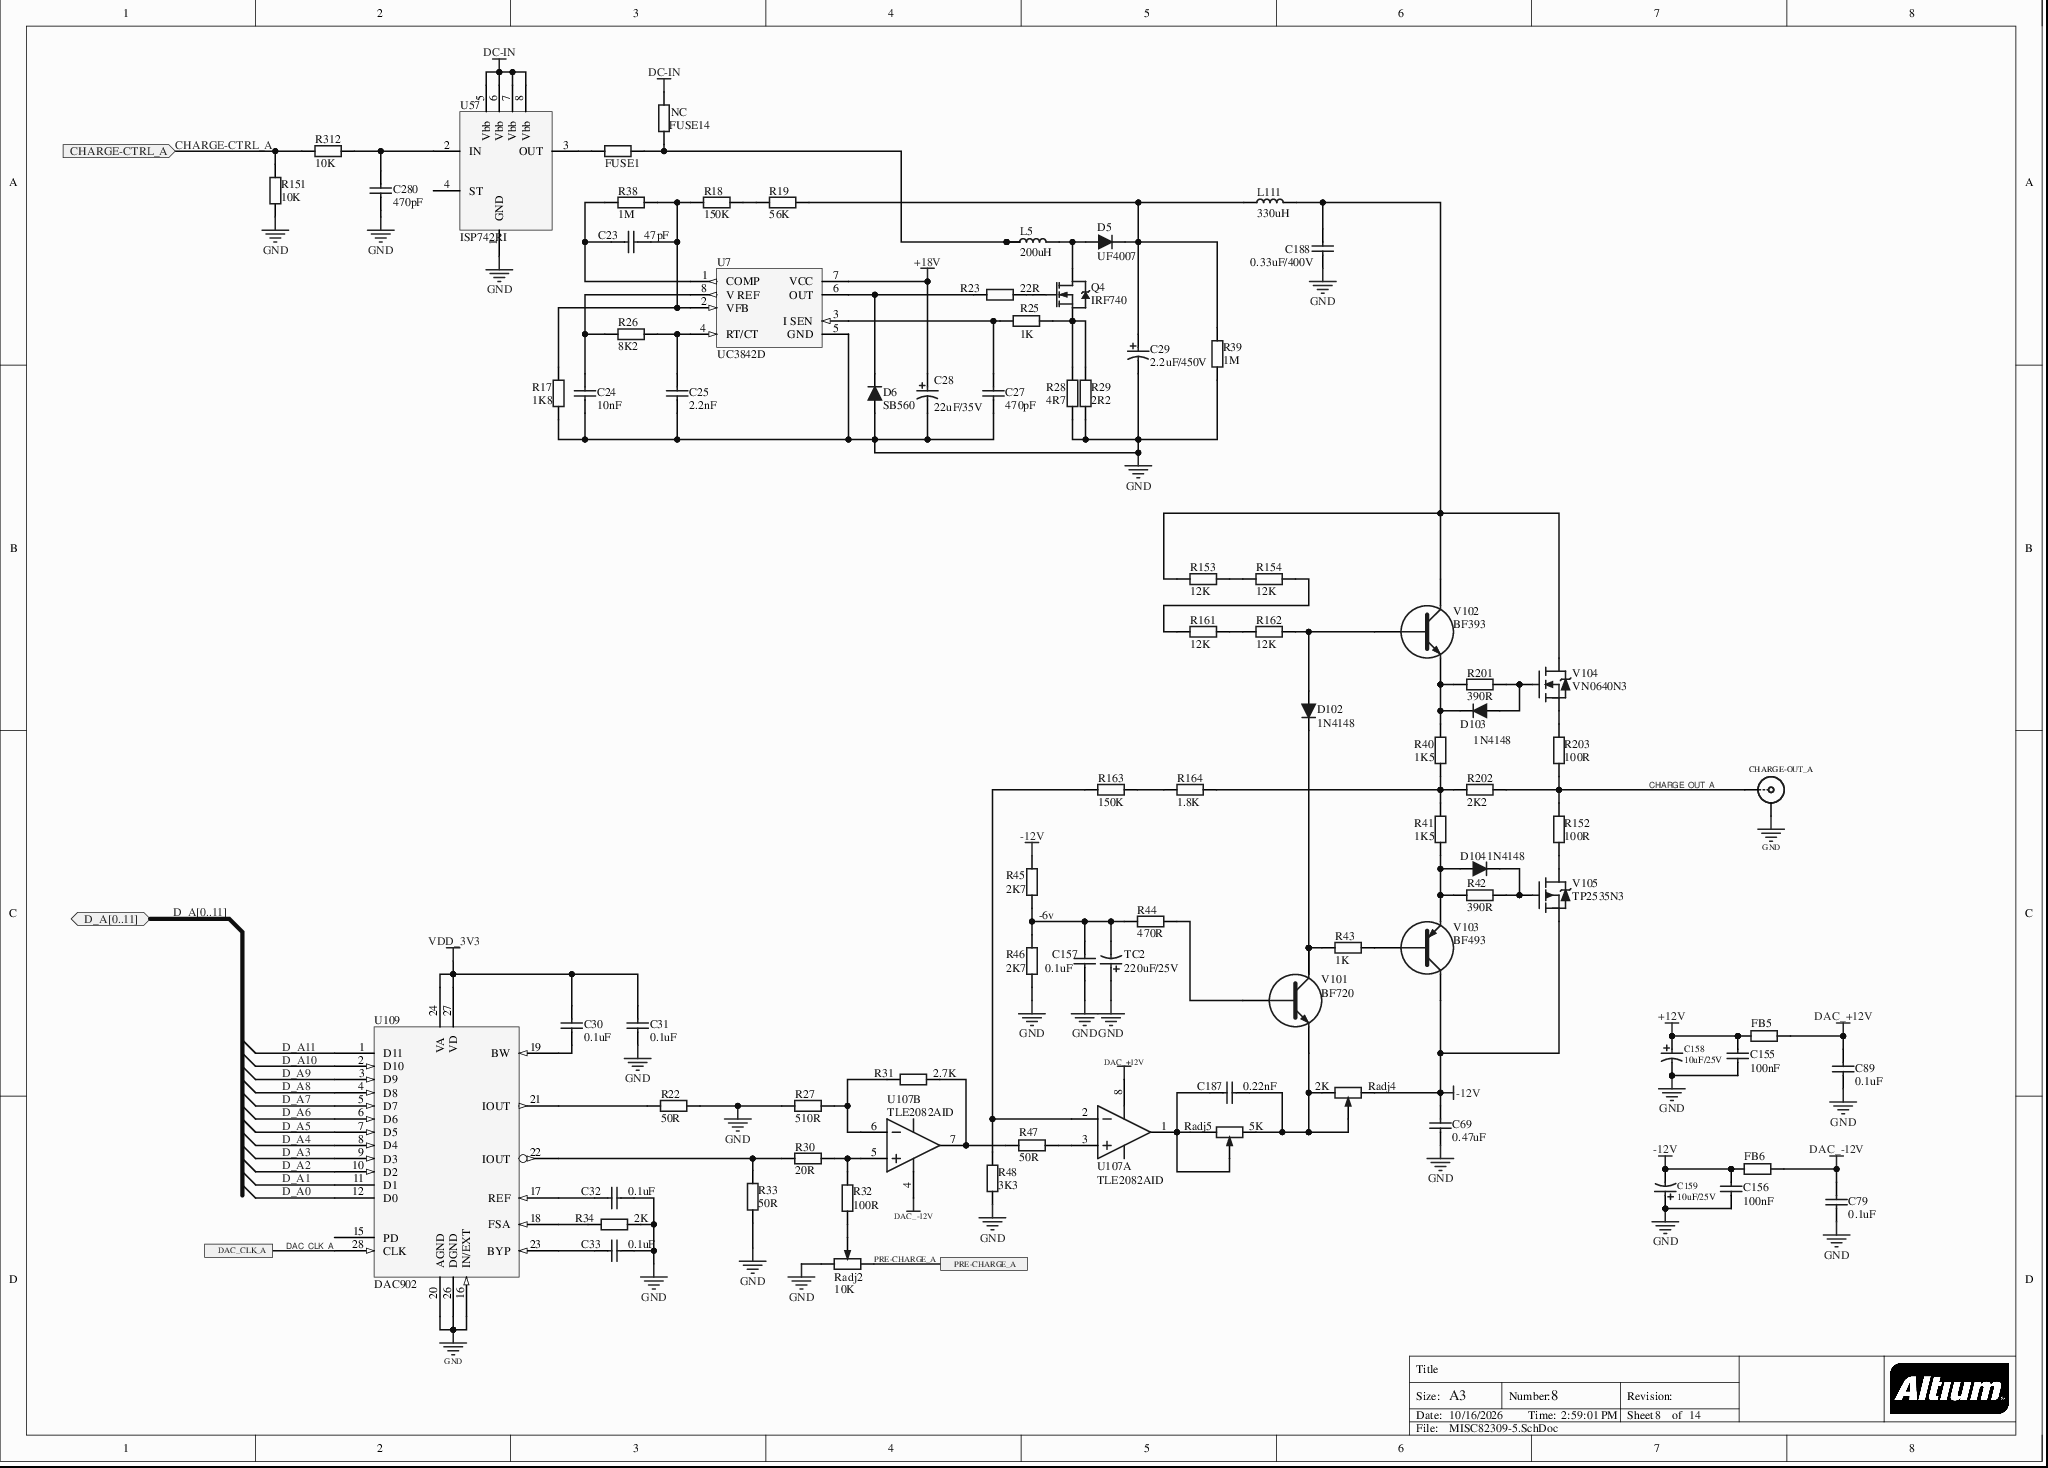
[diagram p0: MISC82309-5.SchDoc]
# Altium project MISC82309-16.PrjPcb (part 4 of 6)

## Sheet MISC82309-5.SchDoc
size A3; DocumentNumber: 8; SheetNumber: 8; SheetTotal: 14

### Parts
C23  47pF  [C1206]
C24  10nF  [C1206]
C25  2.2nF  [C1206]
C27  470pF  [C1206]
C28  22uF/35V  [E6.3X5.4]
C29  2.2uF/450V  [CAP-EL-10X13_5-5]
C30  0.1uF  [CAP_0805]
C31  0.1uF  [CAP_0805]
C32  0.1uF  [CAP_0805]
C33  0.1uF  [CAP_0805]
C69  0.47uF  [C1206]
C79  0.1uF  [C0805]
C89  0.1uF  [C0805]
C155  100nF  [C0805]
C156  100nF  [C0805]
C157  0.1uF  [CAP_0805]
C158  10uF/25V  [E5X5.4]
C159  10uF/25V  [E5X5.4]
C187  0.22nF  [CAP_0805]
C188  0.33uF/400V  [CBB-400V-10mm]
C280  470pF  [C0603]
CHARGE-OUT_A  SMB  [SMB_V-RJ45]  (value not drawn)
D5  UF4007  [DO-41 - 10.46mm]
D6  SB560  [SB560]
D102  1N4148  [DO-213AA]
D103  1N4148  [DO-213AA]
D104  1N4148  [DO-213AA]
FB5  60  [SMD0805-L]  (value not drawn)
FB6  60  [SMD0805-L]  (value not drawn)
FUSE1  ASMD050-1812(30V,0.5A)  [SMD1812-Fuse]  (value not drawn)
FUSE14  value NC  [SMD1812-Fuse]  (hidden comment: ASMD050-1812(30V,0.5A))
L5  200uH  [L200/1.4A]
L111  330uH  [L-9x12]
Q4  IRF740  [TO220V1]
R17  1K8  [R1206]
R18  150K  [R1206]
R19  56K  [R1206]
R22  50R  [RES_0805]
R23  22R  [R1206]
R25  1K  [R1206]
R26  8K2  [R1206]
R27  510R  [RES_0805]
R28  4R7  [R1206]
R29  2R2  [R1206]
R30  20R  [RES_0805]
R31  2.7K  [RES_0805]
R32  100R  [RES_0805]
R33  50R  [RES_0805]
R34  2K  [RES_0805]
R38  1M  [R1206]
R39  1M  [R1206]
R40  1K5  [R1206]
R41  1K5  [R1206]
R42  390R  [R1206]
R43  1K  [R1206]
R44  470R  [RES_0805]
R45  2K7  [RES_0805]
R46  2K7  [RES_0805]
R47  50R  [RES_0805]
R48  3K3  [RES_0805]
R151  10K  [R0603]
R152  100R  [R1206]
R153  12K  [R1206]
R154  12K  [R1206]
R161  12K  [R1206]
R162  12K  [R1206]
R163  150K  [R1206]
R164  1.8K  [R1206]
R201  390R  [R1206]
R202  2K2  [R1206]
R203  100R  [R1206]
R312  10K  [R0603]
Radj2  10K  [Radj]
Radj4  2K  [Radj]
Radj5  5K  [Radj]
TC2  220uF/25V  [E8X10,2]
U7  UC3842D  [SOIC-8]
U57  ISP742RI  [P-DSO-8]
U107  TLE2082AID  [SOIC-8]  (parts A,B of 2)
U109  DAC902  [SOP127P1020X265-28N]
V101  BF720  [SOT223]
V102  BF393  [TO-92]
V103  BF493  [TO-92]
V104  VN0640N3  [TO-92]
V105  TP2535N3  [TO-92]

### Ports
CHARGE-CTRL_A (in), D_A[0..11] (bidir), DAC_CLK_A, PRE-CHARGE_A

### Nets
+12V: C155.1 C158.1 FB5.1
+18V: C28.1 U7.7(VCC)
-12V: C69.1 C156.1 C159.2 FB6.1 R45.1 Radj4.3 V103.3(C) V105.3(D)
DAC_+12V: C89.2 FB5.2 U107.8
DAC_-12V: C79.2 FB6.2 U107.4
DC-IN: FUSE14.1 U57.5(Vbb) U57.6(Vbb) U57.7(Vbb) U57.8(Vbb)
GND: C24.2 C25.2 C27.2 C28.2 C29.2 C31.2 C32.2 C33.1 C69.2 C79.1 C89.1 C155.2 C156.2 C157.2 C158.2 C159.1 C188.1 C280.1 CHARGE-OUT_A.2(Y) D6.1 R17.1 R22.2 R27.1 R28.1 R29.1 R33.1 R34.2 R39.1 R46.2 R48.1 R151.1 Radj2.3 TC2.1 U7.5(GND) U57.1(GND) U109.16(IN/EXT) U109.20(AGND) U109.26(DGND)
VDD_3V3: C30.1 C31.1 U109.24(VA) U109.27(VD)
CHARGE-CTRL_A: R151.2 R312.2 ; port CHARGE-CTRL_A
CHARGE_OUT_A: CHARGE-OUT_A.1(X) R152.1 R202.2 R203.2
D_A0: U109.12(D0)
D_A1: U109.11(D1)
D_A2: U109.10(D2)
D_A3: U109.9(D3)
D_A4: U109.8(D4)
D_A5: U109.7(D5)
D_A6: U109.6(D6)
D_A7: U109.5(D7)
D_A8: U109.4(D8)
D_A9: U109.3(D9)
D_A10: U109.2(D10)
D_A11: U109.1(D11)
DAC_CLK_A: U109.28(CLK) ; port DAC_CLK_A
PRE-CHARGE_A: Radj2.1 ; port PRE-CHARGE_A
NetC23_1: C23.1 R17.2 R18.1 R38.2 U7.2(VFB)
NetC23_2: C23.2 R38.1 U7.1(COMP)
NetC24_1: C24.1 R26.1 U7.8(V_REF)
NetC25_1: C25.1 R26.2 U7.4(RT/CT)
NetC27_1: C27.1 R25.1 U7.3(I_SEN)
NetC29_1: C29.1 D5.2 L111.1 R19.2 R39.2
NetC30_2: C30.2 U109.19(BW)
NetC32_1: C32.1 U109.17(REF)
NetC33_2: C33.2 U109.23(BYP)
NetC157_1: C157.1 R44.2 R45.2 R46.1 TC2.2
NetC187_1: C187.1 Radj4.1 Radj4.2 Radj5.3 V101.3(E)
NetC187_2: C187.2 Radj5.1 Radj5.2 U107.1
NetC188_2: C188.2 L111.2 R153.2 V102.3(C) V104.3(D)
NetC280_2: C280.2 R312.1 U57.2(IN)
NetD5_1: D5.1 L5.2 Q4.2(D)
NetD6_2: D6.2 R23.1 U7.6(OUT)
NetD102_1: D102.1 R162.1 V102.2(B)
NetD102_2: D102.2 R43.2 V101.2(C) V101.4(C)
NetD103_1: D103.1 R201.2 V104.2(G)
NetD103_2: D103.2 R40.1 R201.1 V102.1(E)
NetD104_1: D104.1 R41.2 R42.1 V103.1(E)
NetD104_2: D104.2 R42.2 V105.2(G)
NetFUSE1_1: FUSE1.1 U57.3(OUT)
NetFUSE1_2: FUSE1.2 FUSE14.2 L5.1 L5.3
NetQ4_1: Q4.1(G) R23.2
NetQ4_3: Q4.3(S) R25.2 R28.2 R29.2
NetR18_2: R18.2 R19.1
NetR22_1: R22.1 U109.21(IOUT)
NetR27_2: R27.2 R31.1 U107.6
NetR30_1: R30.1 R33.2 U109.22(IOUT)
NetR30_2: R30.2 R32.2 U107.5
NetR31_2: R31.2 R47.1 U107.7
NetR32_1: R32.1 Radj2.2
NetR34_1: R34.1 U109.18(FSA)
NetR40_2: R40.2 R41.1 R164.1 R202.1
NetR43_1: R43.1 V103.2(B)
NetR44_1: R44.1 V101.1(B)
NetR47_2: R47.2 U107.3
NetR48_2: R48.2 R163.2 U107.2
NetR152_2: R152.2 V105.1(S)
NetR153_1: R153.1 R154.2
NetR154_1: R154.1 R161.2
NetR161_1: R161.1 R162.2
NetR163_1: R163.1 R164.2
NetR203_1: R203.1 V104.1(S)

Not connected (* = marked no-connect by the designer): U57 4(ST); U109 15(PD)

### Buses and harness runs
bus D_A[0..11] = port D_A[0..11]

### Notes on the sheet
- (near R45) -6v
- Title
- Size:
- Date:
- A3
- Number:
- Time:
- Revision:
- Sheet
- of
- File:

### Library data of the parts
C23 = CAP_47pF: Capacitor 47pF; Value: 47pF
C24 = CAP_10nF: Capacitor 10nF; Value: 10nF
C25 = CAP_2.2nF: Capacitor 2.2nF; Value: 2.2nF
C27 = CAP_470pF: Capacitor 470pF; Value: 470pF
C28 = CAP_POLAR_22uF_35V: Polar Capacitor 22uF 35V; Value: 22uF/35V
C29 = CAP_POLAR_2.2uF_450V: Polar Capacitor 222uF 450V; Value: 2.2uF/450V
C30-C33 C157 = CAP_0.1uF: Capacitor 0.1uF; Value: 0.1uF
C69 = CAP_0.47uF: Capacitor 0.47uF; Value: 0.47uF
C79 C89 = CAP_1206: Capacitor; value: 0.1uF
C155 = CAP_0.1uF: value: 470pF
C156 C280 = CAP_0.1uF
  C156: value: 100nF
  C280: value: 470pF
C158 C159 = CAP_POLAR_1: Polar Capacitor
C187 = CAP_0.22nF: Capacitor 0.22nF; Value: 0.22nF
C188 = CAP_CBB_0.33uF_400V: CBB Capacitor 0.33uF 400V; Value: 0.33uF/400V
CHARGE-OUT_A = SMB: SMB Straight Connector; LatestRevisionDate: 17-Jul-2002; LatestRevisionNote: Re-released for DXP Platform.; PCB DECAL: SMB_V-RJ45; Comment_1: SMB; Publisher: Altium Limited
FB5 FB6 = FB: Res; value: 10K
FUSE1 = FUSE: Res; Value: 30V/500mA
FUSE14 = FUSE: Res
L5 = Toroidal Inductor
L111 = Power Inductance: Value: 330uH
Q4 = IRF740: HEXFET N-Channel Power MOSFET; Note: Pin 2 is electrically connected to pin 4.; Published: 8-Jun-2000; LatestRevisionDate: 17-Jul-2002; LatestRevisionNote: Re-released for DXP Platform.; DatasheetVersion: PD-9.375H; PackageVersion: Feb-1997; PackageReference: TO-220AB; PackageDescription: TO, Thru-Hole, Vertical, Heatsink Mounted; 3 In-Line Leads; Pitch 2.54 mm; ComponentLink1Description: Manufacturer Link; ComponentLink1URL: http://www.irf.com/; ComponentLink2Description: Datasheet; ComponentLink2URL: http://www.irf.com/product-info/datasheets/data/irf740.pdf; Publisher: Altium Limited
R17 = Res_1K8: Resistance 1.8K; value: 1K8
R18 R163 = Res_150K: Resistance 150K; value: 150K
R19 = Res_68K: Resistance 68K; value: 56K
R22 R33 R47 = Res_50R: Resistance 50R; value: 50R
R23 = Res_22R: Resistance 22R; value: 22R
R25 R43 = Res_1K: Resistance 1K; value: 1K
R26 = Res_8K2: Resistance 8.2K; value: 8K2
R27 R44 = Res_470R: Resistance 470R
  R27: value: 510R
  R44: value: 470R
R28 = Res_4R7: Resistance 4.7R; value: 4R7
R29 = Res_2R2: Resistance 2R2; value: 2R2
R30 R34 = Res_20R: Resistance 20R
  R30: value: 20R
  R34: value: 2K
R31 R164 = Res_2K: Resistance 2K
  R31: value: 2.7K
  R164: value: 1.8K
R32 R152 R203 = Res_100R: Resistance 100R; value: 100R
R38 R39 = Res_1M: Resistance 1M; value: 1M
R40 R41 = Res_1K5: Resistance 1.5K; value: 1K5
R42 R201 = Res_390R: Resistance 390R; value: 390R
R45 R46 = Res_2K7: Resistance 2.7K; value: 2K7
R48 = Res_3K3: Resistance 3.3K; value: 3K3
R151 R312 = Res2: Resistor; Published: 8-Jun-2000; LatestRevisionDate: 17-Jul-2002; LatestRevisionNote: Re-released for DXP Platform.; PackageReference: AXIAL-0.4; Value: 10K; Publisher: Altium Limited
R153 R154 R161 R162 = Res_12K: Resistance 12K; value: 12K
R202 = Res_2K2: Resistance 2.2K; value: 2K2
Radj2 = Res_Adj_10K: Value: 10K
Radj4 = Res_Adj_2K: Value: 2K
Radj5 = Res_Adj_5K: Value: 5K
TC2 = CAP_POLAR_220uF_25V: Polar Capacitor 220uF 25V; Value: 220uF/25V
U7 = UC3842N: Current Mode PWM Controller; PackageReference: SOIC-8
U57 = I742RI
U107 = TLE2082AID: EXCALIBUR HIGH-SPEED JFET-INPUT  OPERATIONAL AMPLIFIERS
V101 = BF720: NPN high-voltage transistors
V102 = BF393: NPN High Voltage Transistor
V103 = BF493: PNP High Voltage Transistor
D6 = SB560: Supplier 1: Newark; Supplier Part Number 1: 05R5713
U109 = DAC902: Supplier 1: Digi-Key; Supplier Part Number 1: DAC902UG4-ND

## Sheet MISC82309-6.SchDoc
size A3; DocumentNumber: 9; Revision: 1.0; SheetNumber: 9; SheetTotal: 14
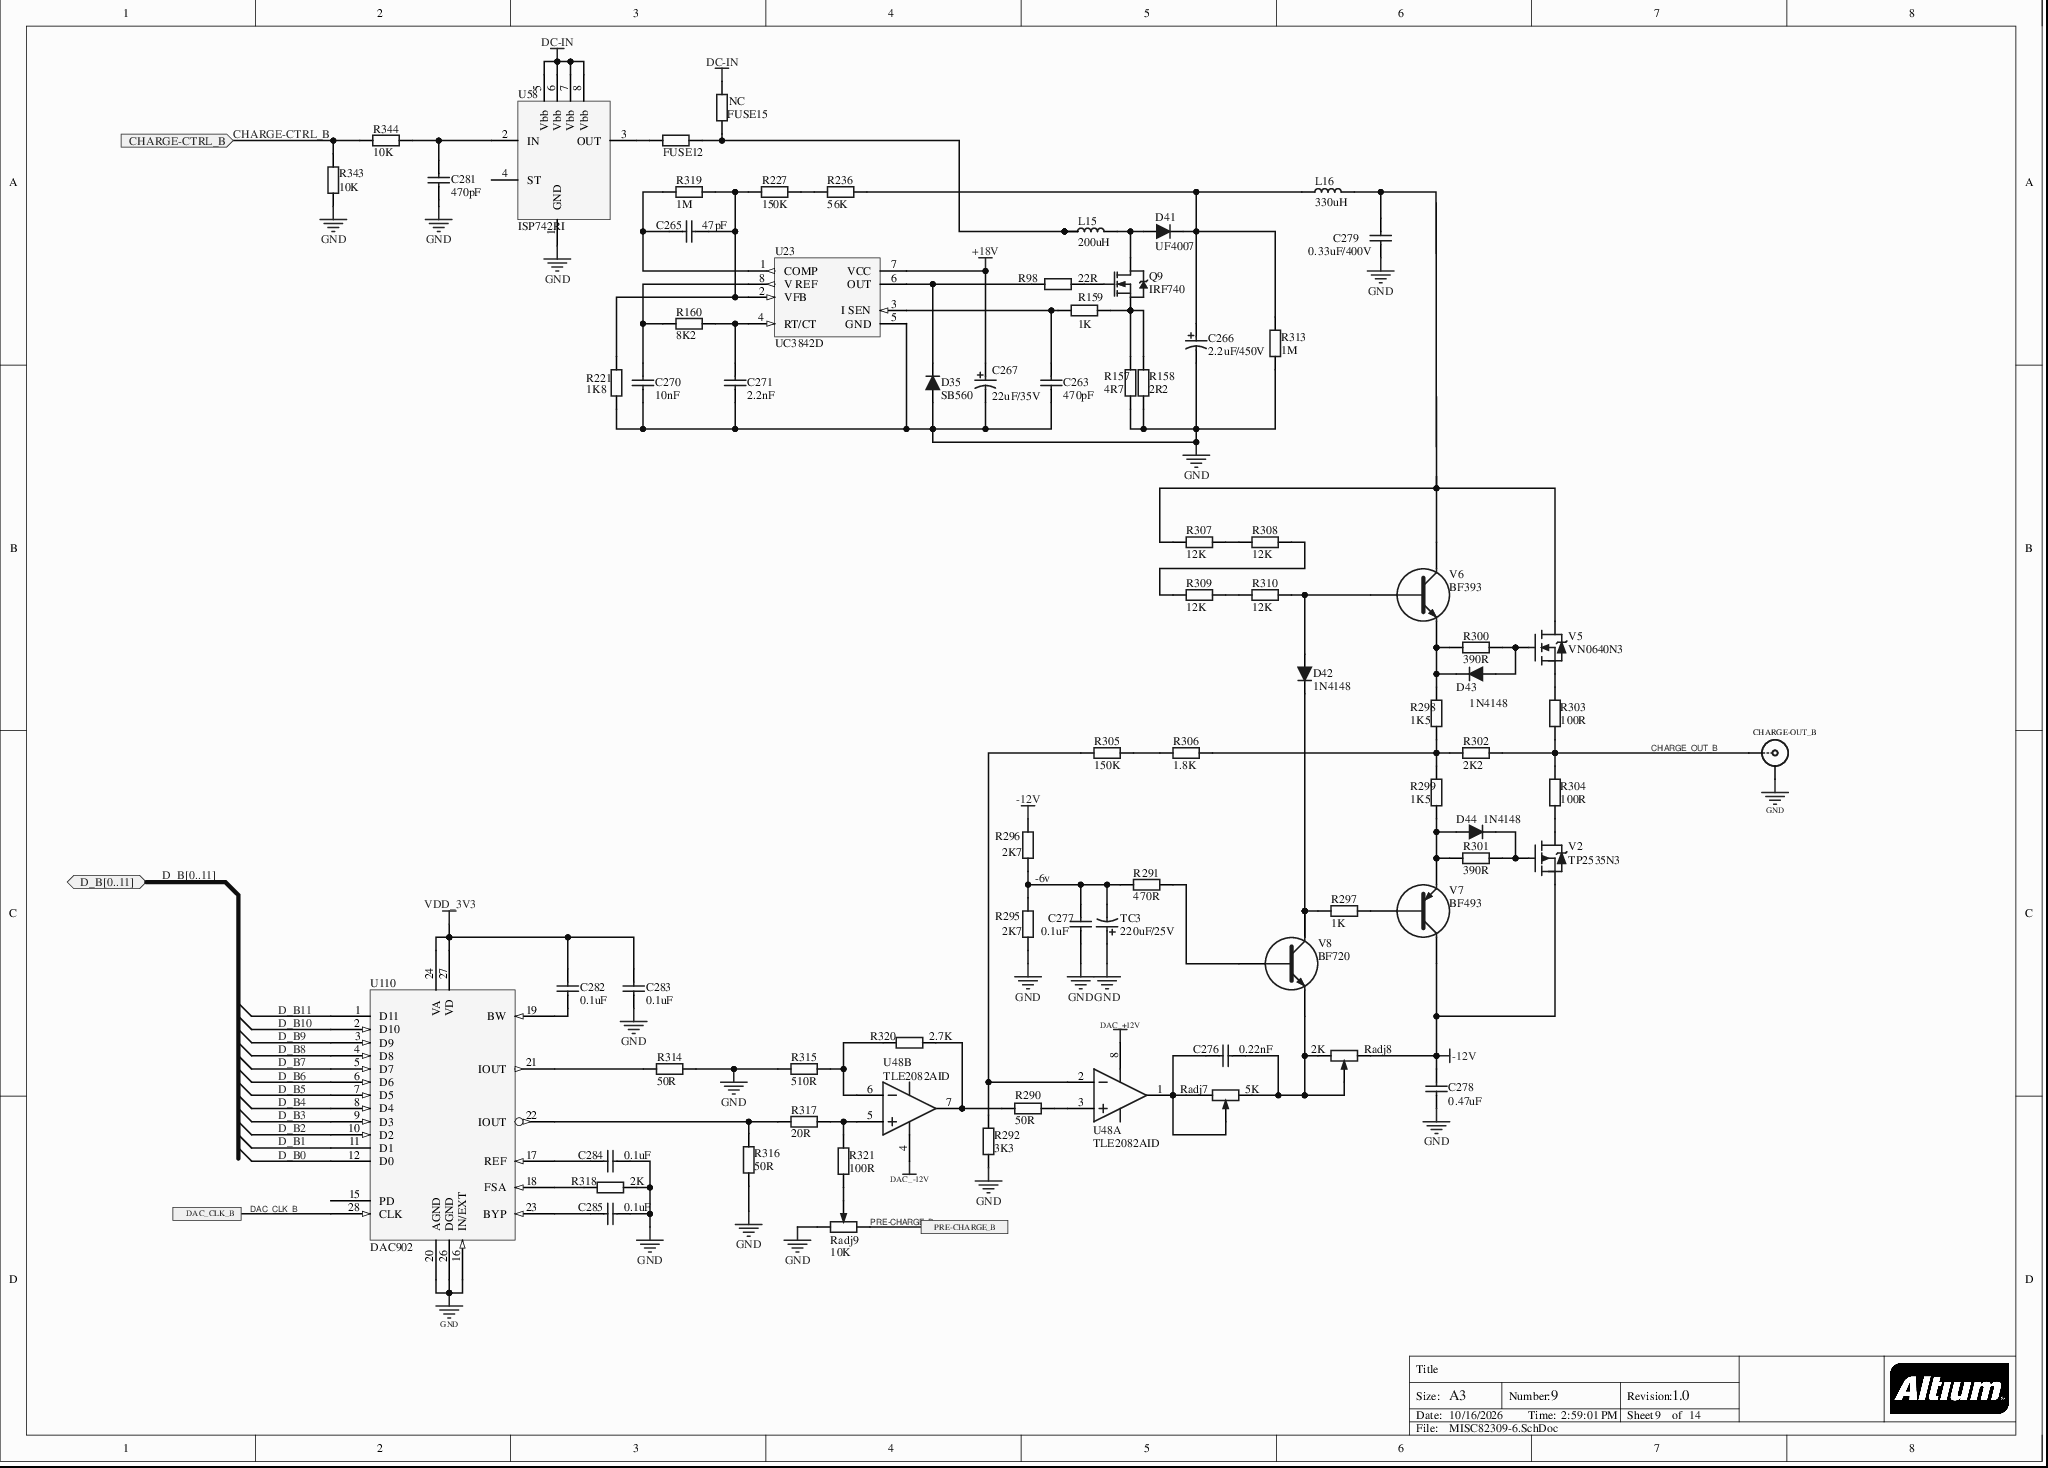
[diagram p1: MISC82309-6.SchDoc]

### Parts
C263  470pF  [C1206]
C265  47pF  [C1206]
C266  2.2uF/450V  [CAP-EL-10X13_5-5]
C267  22uF/35V  [E6.3X5.4]
C270  10nF  [C1206]
C271  2.2nF  [C1206]
C276  0.22nF  [CAP_0805]
C277  0.1uF  [CAP_0805]
C278  0.47uF  [C1206]
C279  0.33uF/400V  [CBB-400V-10mm]
C281  470pF  [C0603]
C282  0.1uF  [CAP_0805]
C283  0.1uF  [CAP_0805]
C284  0.1uF  [CAP_0805]
C285  0.1uF  [CAP_0805]
CHARGE-OUT_B  SMB  [SMB_V-RJ45]  (value not drawn)
D35  SB560  [SB560]
D41  UF4007  [DO-41 - 10.46mm]
D42  1N4148  [DO-213AA]
D43  1N4148  [DO-213AA]
D44  1N4148  [DO-213AA]
FUSE12  ASMD050-1812(30V,0.5A)  [SMD1812-Fuse]  (value not drawn)
FUSE15  value NC  [SMD1812-Fuse]  (hidden comment: ASMD050-1812(30V,0.5A))
L15  200uH  [L200/1.4A]
L16  330uH  [L-9x12]
Q9  IRF740  [TO220V1]
R98  22R  [R1206]
R157  4R7  [R1206]
R158  2R2  [R1206]
R159  1K  [R1206]
R160  8K2  [R1206]
R221  1K8  [R1206]
R227  150K  [R1206]
R236  56K  [R1206]
R290  50R  [RES_0805]
R291  470R  [RES_0805]
R292  3K3  [RES_0805]
R295  2K7  [RES_0805]
R296  2K7  [RES_0805]
R297  1K  [R1206]
R298  1K5  [R1206]
R299  1K5  [R1206]
R300  390R  [R1206]
R301  390R  [R1206]
R302  2K2  [R1206]
R303  100R  [R1206]
R304  100R  [R1206]
R305  150K  [R1206]
R306  1.8K  [R1206]
R307  12K  [R1206]
R308  12K  [R1206]
R309  12K  [R1206]
R310  12K  [R1206]
R313  1M  [R1206]
R314  50R  [RES_0805]
R315  510R  [RES_0805]
R316  50R  [RES_0805]
R317  20R  [RES_0805]
R318  2K  [RES_0805]
R319  1M  [R1206]
R320  2.7K  [RES_0805]
R321  100R  [RES_0805]
R343  10K  [R0603]
R344  10K  [R0603]
Radj7  5K  [Radj]
Radj8  2K  [Radj]
Radj9  10K  [Radj]
TC3  220uF/25V  [E8X10,2]
U23  UC3842D  [SOIC-8]
U48  TLE2082AID  [SOIC-8]  (parts A,B of 2)
U58  ISP742RI  [P-DSO-8]
U110  DAC902  [SOP127P1020X265-28N]
V2  TP2535N3  [TO-92]
V5  VN0640N3  [TO-92]
V6  BF393  [TO-92]
V7  BF493  [TO-92]
V8  BF720  [SOT223]

### Ports
CHARGE-CTRL_B (in), D_B[0..11] (bidir), DAC_CLK_B, PRE-CHARGE_B

### Nets
+18V: C267.1 U23.7(VCC)
-12V: C278.1 R296.1 Radj8.3 V2.3(D) V7.3(C)
DAC_+12V: U48.8
DAC_-12V: U48.4
DC-IN: FUSE15.1 U58.5(Vbb) U58.6(Vbb) U58.7(Vbb) U58.8(Vbb)
GND: C263.2 C266.2 C267.2 C270.2 C271.2 C277.2 C278.2 C279.1 C281.1 C283.2 C284.2 C285.1 CHARGE-OUT_B.2(Y) D35.1 R157.1 R158.1 R221.1 R292.1 R295.2 R313.1 R314.2 R315.1 R316.1 R318.2 R343.1 Radj9.3 TC3.1 U23.5(GND) U58.1(GND) U110.16(IN/EXT) U110.20(AGND) U110.26(DGND)
VDD_3V3: C282.1 C283.1 U110.24(VA) U110.27(VD)
CHARGE-CTRL_B: R343.2 R344.2 ; port CHARGE-CTRL_B
CHARGE_OUT_B: CHARGE-OUT_B.1(X) R302.2 R303.2 R304.1
D_B0: U110.12(D0)
D_B1: U110.11(D1)
D_B2: U110.10(D2)
D_B3: U110.9(D3)
D_B4: U110.8(D4)
D_B5: U110.7(D5)
D_B6: U110.6(D6)
D_B7: U110.5(D7)
D_B8: U110.4(D8)
D_B9: U110.3(D9)
D_B10: U110.2(D10)
D_B11: U110.1(D11)
DAC_CLK_B: U110.28(CLK) ; port DAC_CLK_B
PRE-CHARGE_B: Radj9.1 ; port PRE-CHARGE_B
NetC263_1: C263.1 R159.1 U23.3(I_SEN)
NetC265_1: C265.1 R221.2 R227.1 R319.2 U23.2(VFB)
NetC265_2: C265.2 R319.1 U23.1(COMP)
NetC266_1: C266.1 D41.2 L16.1 R236.2 R313.2
NetC270_1: C270.1 R160.1 U23.8(V_REF)
NetC271_1: C271.1 R160.2 U23.4(RT/CT)
NetC276_1: C276.1 Radj7.3 Radj8.1 Radj8.2 V8.3(E)
NetC276_2: C276.2 Radj7.1 Radj7.2 U48.1
NetC277_1: C277.1 R291.2 R295.1 R296.2 TC3.2
NetC279_2: C279.2 L16.2 R307.2 V5.3(D) V6.3(C)
NetC281_2: C281.2 R344.1 U58.2(IN)
NetC282_2: C282.2 U110.19(BW)
NetC284_1: C284.1 U110.17(REF)
NetC285_2: C285.2 U110.23(BYP)
NetD35_2: D35.2 R98.1 U23.6(OUT)
NetD41_1: D41.1 L15.2 Q9.2(D)
NetD42_1: D42.1 R310.1 V6.2(B)
NetD42_2: D42.2 R297.2 V8.2(C) V8.4(C)
NetD43_1: D43.1 R300.2 V5.2(G)
NetD43_2: D43.2 R298.1 R300.1 V6.1(E)
NetD44_1: D44.1 R299.2 R301.1 V7.1(E)
NetD44_2: D44.2 R301.2 V2.2(G)
NetFUSE12_1: FUSE12.1 U58.3(OUT)
NetFUSE12_2: FUSE12.2 FUSE15.2 L15.1 L15.3
NetQ9_1: Q9.1(G) R98.2
NetQ9_3: Q9.3(S) R157.2 R158.2 R159.2
NetR227_2: R227.2 R236.1
NetR290_1: R290.1 R320.2 U48.7
NetR290_2: R290.2 U48.3
NetR291_1: R291.1 V8.1(B)
NetR292_2: R292.2 R305.2 U48.2
NetR297_1: R297.1 V7.2(B)
NetR298_2: R298.2 R299.1 R302.1 R306.1
NetR303_1: R303.1 V5.1(S)
NetR304_2: R304.2 V2.1(S)
NetR305_1: R305.1 R306.2
NetR307_1: R307.1 R308.2
NetR308_1: R308.1 R309.2
NetR309_1: R309.1 R310.2
NetR314_1: R314.1 U110.21(IOUT)
NetR315_2: R315.2 R320.1 U48.6
NetR316_2: R316.2 R317.1 U110.22(IOUT)
NetR317_2: R317.2 R321.2 U48.5
NetR318_1: R318.1 U110.18(FSA)
NetR321_1: R321.1 Radj9.2

Not connected (* = marked no-connect by the designer): U58 4(ST); U110 15(PD)

### Buses and harness runs
bus D_B[0..11] = port D_B[0..11]

### Notes on the sheet
- (near R296) -6v
- Title
- Size:
- Date:
- A3
- Number:
- Time:
- Revision:
- Sheet
- of
- File:

### Library data of the parts
C263 = CAP_470pF: Capacitor 470pF; Value: 470pF
C265 = CAP_47pF: Capacitor 47pF; Value: 47pF
C266 = CAP_POLAR_2.2uF_450V: Polar Capacitor 222uF 450V; Value: 2.2uF/450V
C267 = CAP_POLAR_22uF_35V: Polar Capacitor 22uF 35V; Value: 22uF/35V
C270 = CAP_10nF: Capacitor 10nF; Value: 10nF
C271 = CAP_2.2nF: Capacitor 2.2nF; Value: 2.2nF
C276 = CAP_0.22nF: Capacitor 0.22nF; Value: 0.22nF
C277 C282-C285 = CAP_0.1uF: Capacitor 0.1uF; Value: 0.1uF
C278 = CAP_0.47uF: Capacitor 0.47uF; Value: 0.47uF
C279 = CAP_CBB_0.33uF_400V: CBB Capacitor 0.33uF 400V; Value: 0.33uF/400V
C281 = CAP_0.1uF: value: 470pF
CHARGE-OUT_B = SMB: SMB Straight Connector; LatestRevisionDate: 17-Jul-2002; LatestRevisionNote: Re-released for DXP Platform.; PCB DECAL: SMB_V-RJ45; Comment_1: SMB; Publisher: Altium Limited
FUSE12 = FUSE: Res; Value: 30V/500mA
FUSE15 = FUSE: Res
L15 = Toroidal Inductor
L16 = Power Inductance: Value: 330uH
Q9 = IRF740: as Q4 on sheet MISC82309-5; Published: 8-Jun-2000; LatestRevisionDate: 17-Jul-2002; LatestRevisionNote: Re-released for DXP Platform.; DatasheetVersion: PD-9.375H; PackageVersion: Feb-1997; PackageReference: TO-220AB; PackageDescription: TO, Thru-Hole, Vertical, Heatsink Mounted; 3 In-Line Leads; Pitch 2.54 mm; ComponentLink1Description: Manufacturer Link; ComponentLink1URL: http://www.irf.com/; ComponentLink2Description: Datasheet; ComponentLink2URL: http://www.irf.com/product-info/datasheets/data/irf740.pdf; Publisher: Altium Limited
R98 = Res_22R: Resistance 22R; value: 22R
R157 = Res_4R7: Resistance 4.7R; value: 4R7
R158 = Res_2R2: Resistance 2R2; value: 2R2
R159 R297 = Res_1K: Resistance 1K; value: 1K
R160 = Res_8K2: Resistance 8.2K; value: 8K2
R221 = Res_1K8: Resistance 1.8K; value: 1K8
R227 R305 = Res_150K: Resistance 150K; value: 150K
R236 = Res_68K: Resistance 68K; value: 56K
R290 R314 R316 = Res_50R: Resistance 50R; value: 50R
R291 R315 = Res_470R: Resistance 470R
  R291: value: 470R
  R315: value: 510R
R292 = Res_3K3: Resistance 3.3K; value: 3K3
R295 R296 = Res_2K7: Resistance 2.7K; value: 2K7
R298 R299 = Res_1K5: Resistance 1.5K; value: 1K5
R300 R301 = Res_390R: Resistance 390R; value: 390R
R302 = Res_2K2: Resistance 2.2K; value: 2K2
R303 R304 R321 = Res_100R: Resistance 100R; value: 100R
R306 R320 = Res_2K: Resistance 2K
  R306: value: 1.8K
  R320: value: 2.7K
R307-R310 = Res_12K: Resistance 12K; value: 12K
R313 R319 = Res_1M: Resistance 1M; value: 1M
R317 R318 = Res_20R: Resistance 20R
  R317: value: 20R
  R318: value: 2K
R343 R344 = Res2: Resistor; Published: 8-Jun-2000; LatestRevisionDate: 17-Jul-2002; LatestRevisionNote: Re-released for DXP Platform.; PackageReference: AXIAL-0.4; Value: 10K; Publisher: Altium Limited
Radj7 = Res_Adj_5K: Value: 5K
Radj8 = Res_Adj_2K: Value: 2K
Radj9 = Res_Adj_10K: Value: 10K
TC3 = CAP_POLAR_220uF_25V: Polar Capacitor 220uF 25V; Value: 220uF/25V
U23 = UC3842N: Current Mode PWM Controller; PackageReference: SOIC-8
U48 = TLE2082AID: as U107 on sheet MISC82309-5
U58 = I742RI
V6 = BF393: NPN High Voltage Transistor
V7 = BF493: PNP High Voltage Transistor
V8 = BF720: NPN high-voltage transistors
D35 = SB560: Supplier 1: Newark; Supplier Part Number 1: 05R5713
U110 = DAC902: Supplier 1: Digi-Key; Supplier Part Number 1: DAC902UG4-ND

## Sheet MISC82309-3.SchDoc
size A3; DocumentNumber: 10; Revision: 1.0; SheetNumber: 10; SheetTotal: 14
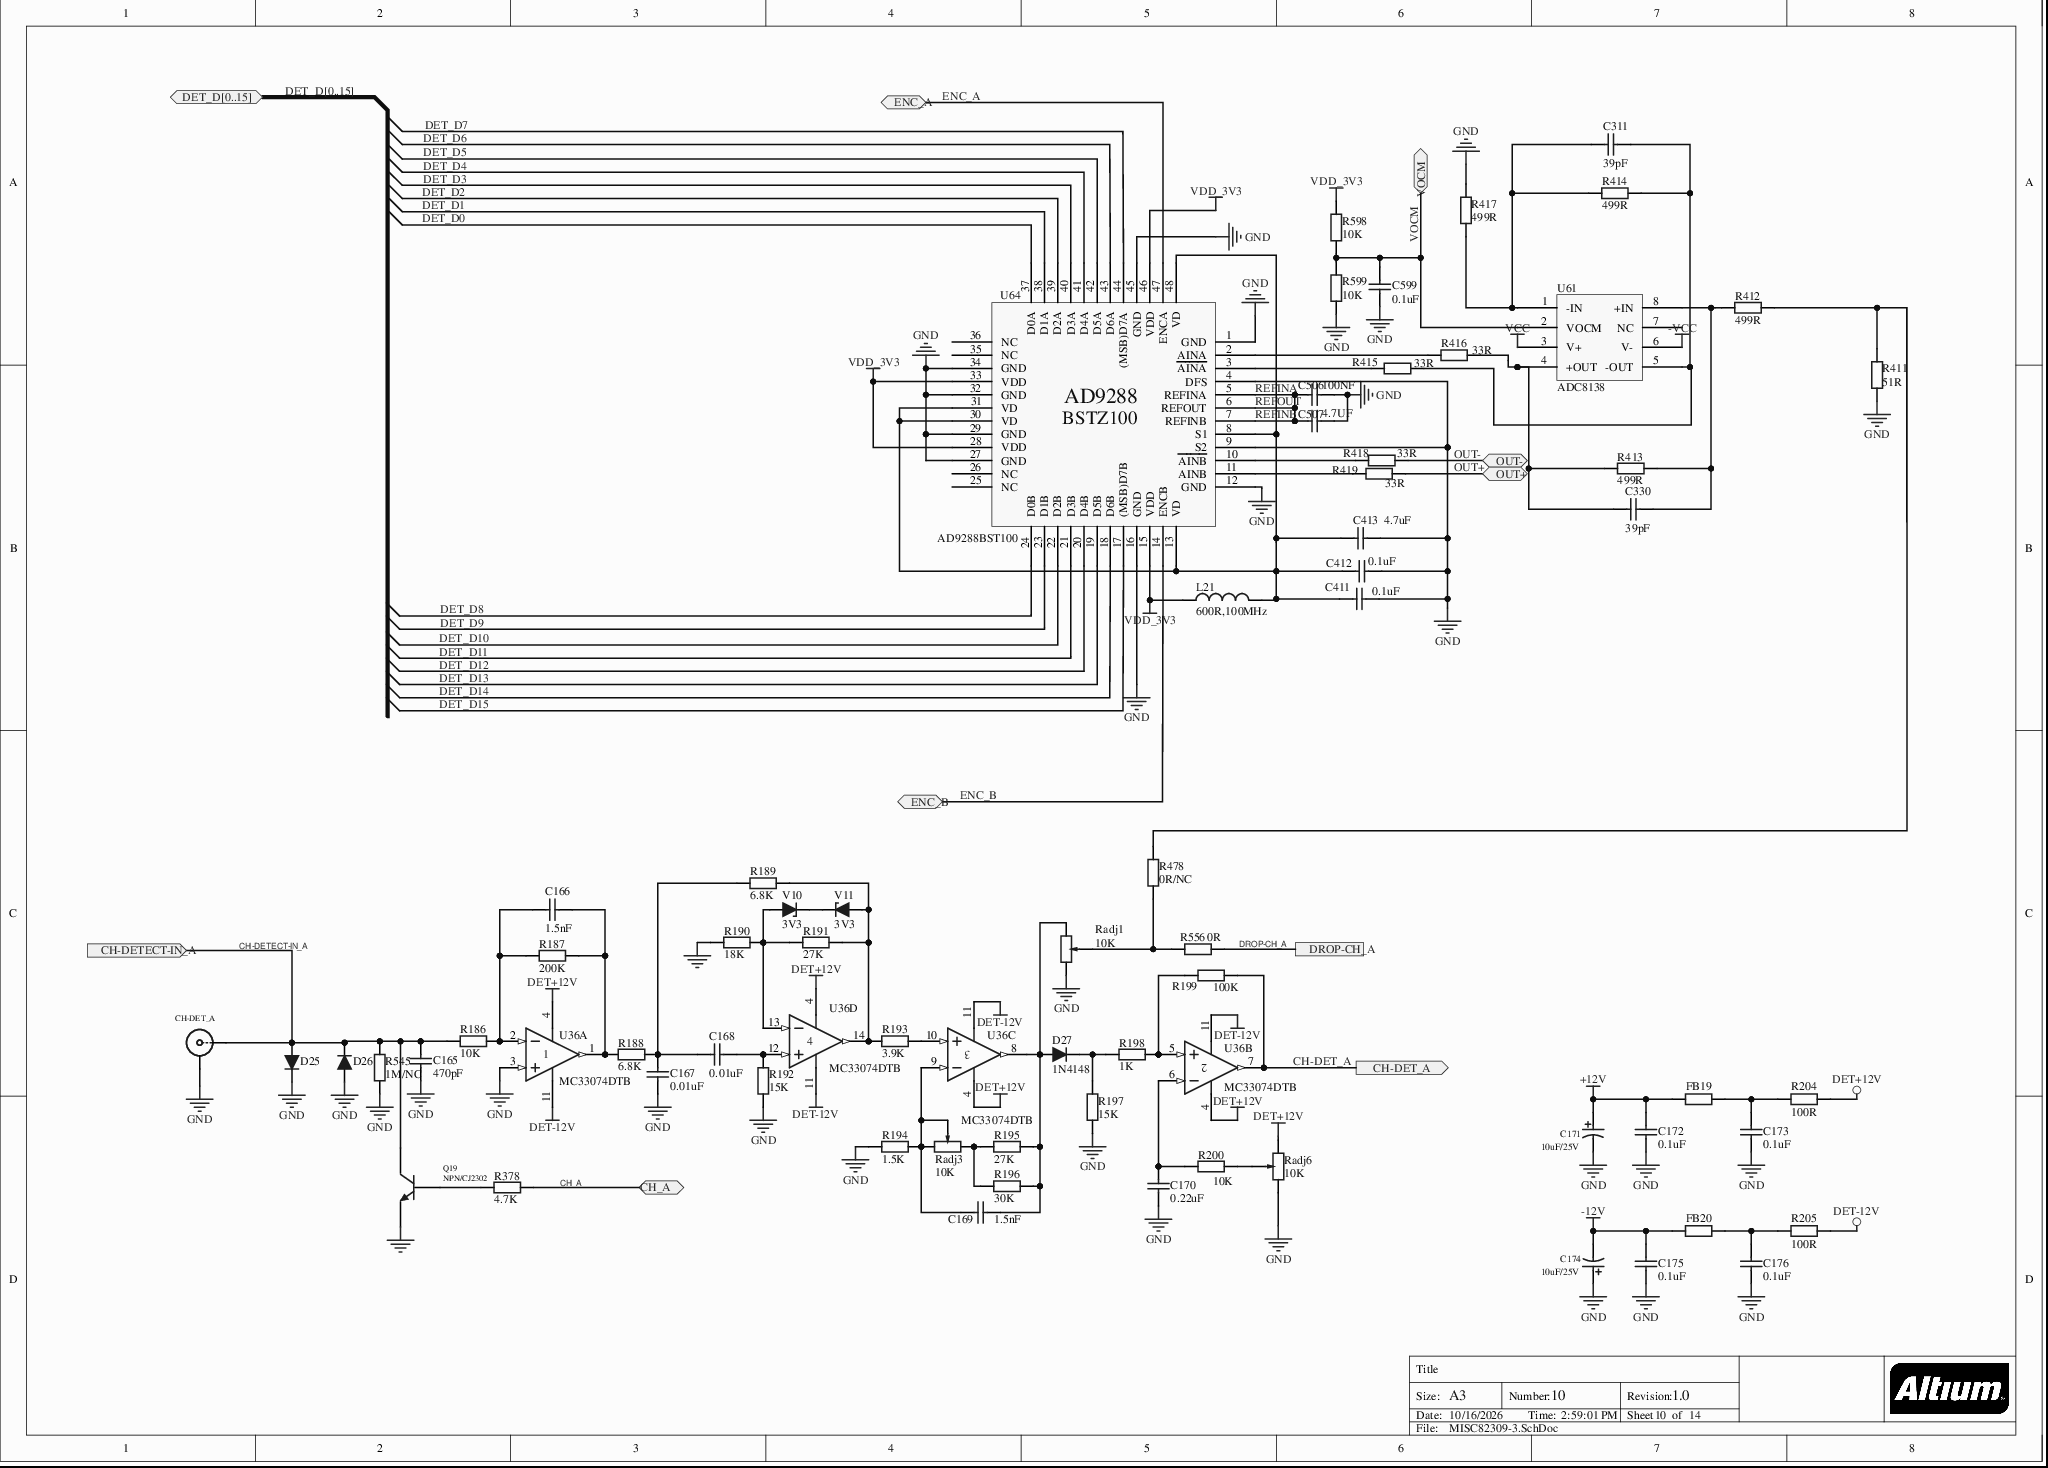
[diagram p2: MISC82309-3.SchDoc]

### Parts
C165  470pF  [C0603]
C166  1.5nF  [C0603]
C167  0.01uF  [C0603]
C168  0.01uF  [C0603]
C169  1.5nF  [C0603]
C170  0.22uF  [C0603]
C171  10uF/25V  [E5X5.4]
C172  0.1uF  [C0805]
C173  0.1uF  [C0805]
C174  10uF/25V  [E5X5.4]
C175  0.1uF  [C0805]
C176  0.1uF  [C0805]
C311  39pF  [CAP_0603]
C330  39pF  [CAP_0603]
C411  0.1uF  [CAP_0603]
C412  0.1uF  [CAP_0603]
C413  4.7uF  [CAP_0603]
C506  value 100NF  [c0603]  (hidden comment: Cap Semi)
C507  value 4.7UF  [c0603]  (hidden comment: Cap Semi)
C599  0.1uF  [CAP_0603]
CH-DET_A  SMB  [SMB_V-RJ45]  (value not drawn)
D25  1N4148WS  [SOD323]  (value not drawn)
D26  1N4148WS  [SOD323]  (value not drawn)
D27  1N4148  [SOD-323]
FB19  60  [SMD0805-L]  (value not drawn)
FB20  60  [SMD0805-L]  (value not drawn)
L21  600R,100MHz  [R0805]
Q19  NPN/CJ2302  [SOT-23-3]
R186  10K  [RES_0603]
R187  200K  [RES_0603]
R188  6.8K  [RES_0603]
R189  6.8K  [RES_0603]
R190  18K  [RES_0603]
R191  27K  [RES_0603]
R192  15K  [RES_0603]
R193  3.9K  [RES_0603]
R194  1.5K  [RES_0603]
R195  27K  [RES_0603]
R196  30K  [RES_0603]
R197  15K  [RES_0603]
R198  1K  [RES_0603]
R199  100K  [RES_0603]
R200  10K  [RES_0603]
R204  100R  [R0805]
R205  100R  [R0805]
R378  4.7K  [RES_0603]
R411  51R  [RES_0603]
R412  499R  [RES_0603]
R413  499R  [RES_0603]
R414  499R  [RES_0603]
R415  33R  [RES_0603]
R416  33R  [RES_0603]
R417  499R  [RES_0603]
R418  33R  [RES_0603]
R419  33R  [RES_0603]
R478  0R/NC  [RES_0603]
R545  1M/NC  [RES_0603]
R556  0R  [RES_0603]
R598  10K  [RES_0603]
R599  10K  [RES_0603]
Radj1  10K  [Radj]
Radj3  10K  [Radj]
Radj6  10K  [Radj]
U36  MC33074DTB  [948G-01_N]  (parts A,B,C,D of 4)
U61  ADC8138  [SO8]
U64  AD9288BST100  [LQFP48A]
V10  3V3  [SOD-123]
V11  3V3  [SOD-123]

### Ports
CH-DET_A (out), CH-DETECT-IN_A (in), CH_A (bidir), DET_D[0..15] (bidir), DROP-CH_A, ENC_A (bidir), ENC_B (bidir), OUT+ (bidir), OUT- (bidir), VOCM (bidir)

### Nets
+12V: C171.1 C172.2 FB19.1
-12V: C174.2 C175.2 FB20.1
-VCC: U61.6(V-)
DET+12V: R204.2 Radj6.3 U36.4(V+)
DET-12V: R205.2 U36.11(V-)
GND: C165.1 C167.2 C170.2 C171.2 C172.1 C173.1 C174.1 C175.1 C176.1 C411.1 C412.1 C413.1 C506.2 C507.2 C599.2 CH-DET_A.2(Y) D25.2 D26.1 Q19.2(E) R190.1 R192.1 R194.1 R197.1 R411.2 R417.2 R545.1 R599.1 Radj1.1 Radj6.1 U36.3(IN+) U64.1(GND) U64.4(DFS) U64.9(S2) U64.12(GND) U64.16(GND) U64.27(GND) U64.29(GND) U64.32(GND) U64.34(GND) U64.45(GND)
VCC: U61.3(V+)
VDD_3V3: L21.2 R598.2 U64.15(VDD) U64.28(VDD) U64.33(VDD) U64.46(VDD)
CH-DET_A: R199.2 U36.7(OUT) ; port CH-DET_A
CH-DETECT-IN_A: C165.2 CH-DET_A.1(X) D25.1 D26.2 Q19.3(C) R186.1 R545.2 ; port CH-DETECT-IN_A
CH_A: R378.2 ; port CH_A
DET_D0: U64.37(D0A)
DET_D1: U64.38(D1A)
DET_D2: U64.39(D2A)
DET_D3: U64.40(D3A)
DET_D4: U64.41(D4A)
DET_D5: U64.42(D5A)
DET_D6: U64.43(D6A)
DET_D7: U64.44((MSB)D7A)
DET_D8: U64.24(D0B)
DET_D9: U64.23(D1B)
DET_D10: U64.22(D2B)
DET_D11: U64.21(D3B)
DET_D12: U64.20(D4B)
DET_D13: U64.19(D5B)
DET_D14: U64.18(D6B)
DET_D15: U64.17((MSB)D7B)
DROP-CH_A: R556.1 ; port DROP-CH_A
ENC_A: U64.47(ENCA) ; port ENC_A
ENC_B: U64.14(ENCB) ; port ENC_B
OUT+: R419.1 ; port OUT+
OUT-: R418.2 ; port OUT-
REFINA: C506.1 C507.1 U64.5(REFINA) U64.6(REFOUT) U64.7(REFINB)  [also labelled REFINB, REFOUT]
VOCM: C599.1 R598.1 R599.2 U61.2(VOCM) ; port VOCM
NetC166_1: C166.1 R187.2 R188.1 U36.1(OUT)
NetC166_2: C166.2 R186.2 R187.1 U36.2(IN-)
NetC167_1: C167.1 C168.2 R188.2 R189.1
NetC168_1: C168.1 R192.2 U36.12(IN+)
NetC169_1: C169.1 D27.1 R195.2 R196.2 Radj1.3 U36.8(OUT)
NetC169_2: C169.2 R194.2 Radj3.2 Radj3.3 U36.9(IN-)
NetC170_1: C170.1 R200.1 U36.6(IN-)
NetC173_2: C173.2 FB19.2 R204.1
NetC176_2: C176.2 FB20.2 R205.1
NetC311_1: C311.1 R414.1 R415.1 U61.5(-OUT)
NetC311_2: C311.2 R414.2 R417.1 U61.1(-IN)
NetC330_1: C330.1 R413.1 R416.2 U61.4(+OUT)
NetC330_2: C330.2 R412.1 R413.2 U61.8(+IN)
NetC411_2: C411.2 C412.2 C413.2 L21.1 U64.8(S1) U64.13(VD) U64.30(VD) U64.31(VD) U64.48(VD)
NetD27_2: D27.2 R197.2 R198.1
NetQ19_1: Q19.1(B) R378.1
NetR189_2: R189.2 R191.2 R193.2 U36.14(OUT) V11.1
NetR190_2: R190.2 R191.1 U36.13(IN-) V10.1
NetR193_1: R193.1 U36.10(IN+)
NetR195_1: R195.1 R196.1 Radj3.1
NetR198_2: R198.2 R199.1 U36.5(IN+)
NetR200_2: R200.2 Radj6.2
NetR411_1: R411.1 R412.2 R478.2
NetR415_2: R415.2 U64.3(~{AINA})
NetR416_1: R416.1 U64.2(AINA)
NetR418_1: R418.1 U64.10(~{AINB})
NetR419_2: R419.2 U64.11(AINB)
NetR478_1: R478.1 R556.2 Radj1.2
NetV10_2: V10.2 V11.2

Not connected (* = marked no-connect by the designer): U61 7(NC); U64 25(NC) 26(NC) 35(NC) 36(NC)

### Buses and harness runs
bus DET_D[0..15] = port DET_D[0..15]

### Notes on the sheet
- Title
- Size:
- Date:
- A3
- Number:
- Time:
- Revision:
- Sheet
- of
- File:

### Library data of the parts
C165-C170 C311 C330 C411-C413 C599 = CAP_0603: Capacitor
  C165: value: 470pF
  C166 C169: value: 1.5nF
  C167 C168: value: 0.01uF
  C170: value: 0.22uF
  C311 C330: value: 39pF
  C411 C412 C599: value: 0.1uF
  C413: value: 4.7uF
C171 C174 = CAP_POLAR_1: Polar Capacitor
C172 C173 C175 C176 = CAP_1206: Capacitor; value: 0.1uF
C506 C507 = Cap Semi: Capacitor (Semiconductor SIM Model); Published: 8-Jun-2000; LatestRevisionDate: 29-May-2009; LatestRevisionNote: IPC-7351 Footprint Added.; PackageReference: C1206; PackageDescription: Chip Capacitor; Publisher: Altium Limited
CH-DET_A = SMB: SMB Straight Connector; LatestRevisionDate: 17-Jul-2002; LatestRevisionNote: Re-released for DXP Platform.; PCB DECAL: SMB_V-RJ45; Comment_1: SMB; Publisher: Altium Limited
D27 = Diode-SMD
FB19 FB20 = FB: Res; value: 10K
L21 = Inductor: value: 600R,100MHz
Q19 = NPN: Value: NPN/CJ2302
R186-R193 R195-R200 R378 R411-R419 R478 R545 R556 R598 R599 = Res_0603: Res
  R186 R200 R598 R599: value: 10K
  R187: value: 200K
  R188 R189: value: 6.8K
  R190: value: 18K
  R191 R195: value: 27K
  R192 R197: value: 15K
  R193: value: 3.9K
  R196: value: 30K
  R198: value: 1K
  R199: value: 100K
  R378: value: 4.7K
  R411: value: 51R
  R412-R414 R417: value: 499R
  R415 R416 R418 R419: value: 33R
  R478: value: 0R/NC
  R545: value: 1M/NC
  R556: value: 0R
R194 = Res_0603: Res; value: 10K
R204 R205 = Res2: Resistor; Published: 8-Jun-2000; LatestRevisionDate: 17-Jul-2002; LatestRevisionNote: Re-released for DXP Platform.; PackageReference: AXIAL-0.4; Value: 100R; Publisher: Altium Limited
Radj1 Radj3 Radj6 = Radj: value: 10K
U36 = MC33074DTB: Single-Supply 3 to 44 V Operational Amplifier; Published: 28-Feb-2003; LatestRevisionDate: 12-Dec-2006; LatestRevisionNote: IPC-7351 Footprint Added.; DatasheetVersion: Jan-2002, Rev. 5; PackageVersion: 1998; PackageReference: 948G-01; PackageDescription: 14-Pin Thin Small Outline Package 0.65 mm Pitch; ComponentLink1Description: Manufacturer Link; ComponentLink1URL: http://www.onsemi.com/; ComponentLink2Description: Datasheet; ComponentLink2URL: http://www.onsemi.com/pub/Collateral/MC34071-D.PDF; Publisher: Altium Limited
U61 = AD8138
U64 = AD9288
V10 V11 = BZT52C3V3